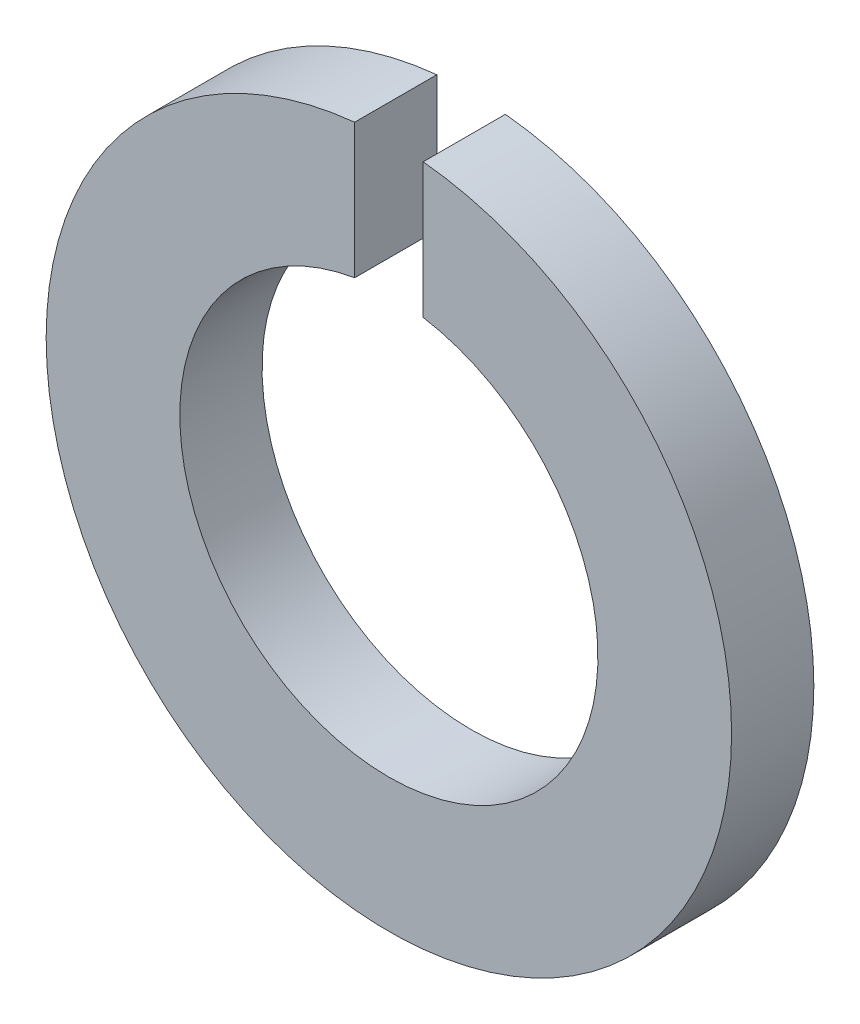
from build123d import *

# Parameters (mm, degrees)
BOSS_EXTRUDE1_DEPTH = 1.2


with BuildPart() as part:
    # Sketch1 → Boss-Extrude1 (new body)
    with BuildSketch(Plane.XY.offset(229.899812353)):
        with BuildLine():
            Line((0.5, 4.974937186), (0.5, 3.008737277))
            ThreePointArc((0.5, 3.008737277), (0, -3.05), (-0.5, 3.008737277))
            Line((-0.5, 3.008737277), (-0.5, 4.974937186))
            ThreePointArc((-0.5, 4.974937186), (0, -5), (0.5, 4.974937186))
        make_face()
    extrude(amount=-BOSS_EXTRUDE1_DEPTH)


solid = part.part
